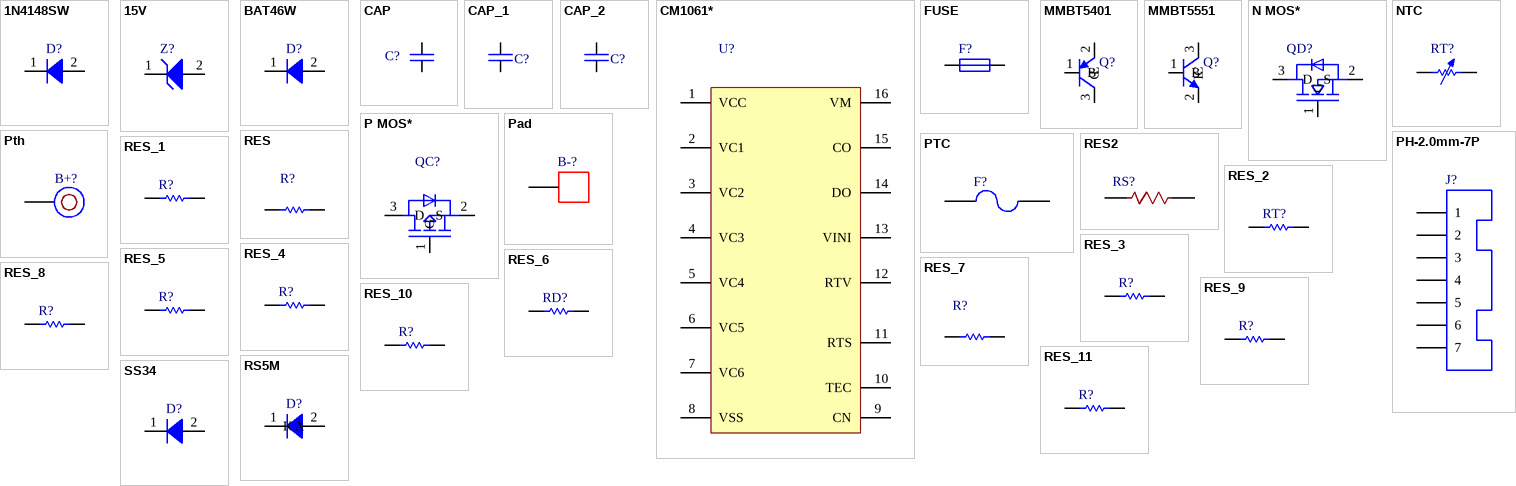
[diagram p0: symbols 1N4148SW to SS34]
# Altium schematic symbol library MISC75736.SCHLIB: 32 symbols
Pins are listed as number, name and electrical type; pins without a type are passive.


## 1N4148SW
designator D?
chip diode
footprint SOD123 (chip diode)
footprint SOD323 (chip diode)
pins: 1 A, 2    

## 15V
designator Z?
chip Zener diode
footprint SOD123 (chip diode)
footprint SOD323 (chip diode)
pins: 1 A, 2 K

## BAT46W
designator D?
chip diode
footprint SOD123 (chip diode)
footprint SOD323 (chip diode)
footprint SMAF
footprint SMC (chip diode)
pins: 1 A, 2 K

## CAP
designator C?
chip capacitor
footprint C0402A (chip capacitor)
footprint C0603A (chip capacitor)
footprint C0402L (chip resistor)
footprint C0805A (chip capacitor)
footprint C1206A (chip capacitor)
footprint C0603L (chip J-type capacitor)
footprint C0805L (chip capacitor)
footprint C0603M (chip capacitor)
pins: 1, 2

## CAP_1
designator C?
chip capacitor
footprint C0402A (chip capacitor)
footprint C0603A (chip capacitor)
footprint C0402L (chip resistor)
footprint C0805A (chip capacitor)
footprint C1206A (chip capacitor)
footprint C0603L (chip J-type capacitor)
footprint C0805L (chip capacitor)
footprint C0603M (chip capacitor)
pins: 1, 2

## CAP_2
designator C?
chip capacitor
footprint C0402A (chip capacitor)
footprint C0603A (chip capacitor)
footprint C0402L (chip resistor)
footprint C0805A (chip capacitor)
footprint C1206A (chip capacitor)
footprint C0603L (chip J-type capacitor)
footprint C0805L (chip capacitor)
footprint C0603M (chip capacitor)
pins: 1, 2

## CM1061*
designator U?
6-cell battery protection IC
footprint SOP16L
pins: 1 VCC, 2 VC1, 3 VC2, 4 VC3, 5 VC4, 6 VC5, 7 VC6, 8 VSS, 9 CN, 10 TEC, 11 RTS, 12 RTV, 13 VINI, 14 DO, 15 CO, 16 VM

## FUSE
designator F?
footprint R1206A (chip resistor)
footprint R0603A (chip resistor)
footprint R0805A (chip resistor)
footprint F2410 (chip fuse)
footprint J10*3mm (jumper 10*3mm)
pins: 1, 2

## MMBT5401
designator Q?
chip transistor
footprint SOT23-3 (chip IC/MOS*)
footprint SOT23-3L (chip MOS)
footprint SOT23-3 (chip IC/MOS*)
pins: 1 B, 2 E, 3 C

## MMBT5551
designator Q?
chip transistor
footprint SOT23-3 (chip IC/MOS*)
footprint SOT23-3L (chip MOS)
pins: 1 B, 2 E, 3 C

## N MOS*
designator QD?
chip MOSFET
footprint TO-252
footprint TO-252-DFN
footprint DFN5X6(T3)
footprint SOP-8L(T3p)
footprint DFN5X6(T3p) (chip MOS (non-standard))
footprint TO-263-TOLL
footprint DFN-3x3
footprint DFN-3x3L8(T3P) (chip MOSFET)
footprint TOLL_123 (chip MOSFET)
footprint TOLL_GSD (chip MOSFET)
pins: 1 G, 2 S, 3 D

## NTC
designator RT?
chip thermistor
footprint R0603A (chip resistor)
footprint R0402A (chip resistor)
footprint RT2.3X1-2 (wire-bond NTC)
footprint R0603L (chip resistor)
footprint R0603m (chip resistor)
footprint RT2.3X1.2-2 (wire-bond NTC)
pins: 1, 2

## P MOS*
designator QC?
chip MOSFET
footprint TOLL (chip MOSFET)
footprint TO-252
footprint TO-252-DFN
footprint DFN5X6(T3)
footprint SOP-8L(T3p)
footprint DFN5X6(T3p) (chip MOS (non-standard))
footprint TO-263-TOLL
pins: 1 G, 2 S, 3 D

## Pad
designator B-?
connection pad (non-through-hole)
footprint 3*3
footprint Pad10X8mm
footprint Pad8X6mm
pins: 1

## PH-2.0mm-7P
designator J?
connector
pins: 1, 2, 3, 4, 5, 6, 7

## PTC
designator F?
chip resettable fuse
footprint F1812A (chip resistor)
pins: 1, 2

## Pth
designator B+?
through-hole pad
footprint 4*3 (through-hole pad)
pins: 1

## RES
designator R?
chip resistor
footprint R0603A (chip resistor)
footprint R0201A
footprint R0402A (chip resistor)
footprint R0603m (chip resistor)
footprint R0805A (chip resistor)
footprint R0402L (chip resistor)
footprint RES0603 (CAP0402)
footprint R0603L (chip resistor)
footprint R0805L (chip resistor)
footprint R0805M (chip resistor)
footprint R1206A (chip resistor)
pins: 1, 2

## RES2
designator RS?
chip metal alloy resistor
footprint R2512L (chip resistor)
pins: 1, 2

## RES_1
designator R?
chip resistor
footprint R0603A (chip resistor)
footprint R0201A
footprint R0402A (chip resistor)
footprint R0603m (chip resistor)
footprint R0805A (chip resistor)
footprint R0402L (chip resistor)
footprint RES0603 (CAP0402)
footprint R0603L (chip resistor)
footprint R0805L (chip resistor)
footprint R0805M (chip resistor)
footprint R1206A (chip resistor)
pins: 1, 2

## RES_2
designator RT?
chip resistor
footprint R0603A (chip resistor)
footprint R0201A
footprint R0402A (chip resistor)
footprint R0603m (chip resistor)
footprint R0805A (chip resistor)
footprint R0402L (chip resistor)
footprint RES0603 (CAP0402)
footprint R0603L (chip resistor)
footprint R0805L (chip resistor)
footprint R0805M (chip resistor)
footprint R1206A (chip resistor)
pins: 1, 2

## RES_3
designator R?
chip resistor
footprint R0603A (chip resistor)
footprint R0201A
footprint R0402A (chip resistor)
footprint R0603m (chip resistor)
footprint R0805A (chip resistor)
footprint R0402L (chip resistor)
footprint RES0603 (CAP0402)
footprint R0603L (chip resistor)
footprint R0805L (chip resistor)
footprint R0805M (chip resistor)
footprint R1206A (chip resistor)
pins: 1, 2

## RES_4
designator R?
chip resistor
footprint R0603A (chip resistor)
footprint R0201A
footprint R0402A (chip resistor)
footprint R0603m (chip resistor)
footprint R0805A (chip resistor)
footprint R0402L (chip resistor)
footprint RES0603 (CAP0402)
footprint R0603L (chip resistor)
footprint R0805L (chip resistor)
footprint R0805M (chip resistor)
footprint R1206A (chip resistor)
pins: 1, 2

## RES_5
designator R?
chip resistor
footprint R0603A (chip resistor)
footprint R0201A
footprint R0402A (chip resistor)
footprint R0603m (chip resistor)
footprint R0805A (chip resistor)
footprint R0402L (chip resistor)
footprint RES0603 (CAP0402)
footprint R0603L (chip resistor)
footprint R0805L (chip resistor)
footprint R0805M (chip resistor)
footprint R1206A (chip resistor)
pins: 1, 2

## RES_6
designator RD?
chip resistor
footprint R0603A (chip resistor)
footprint R0201A
footprint R0402A (chip resistor)
footprint R0603m (chip resistor)
footprint R0805A (chip resistor)
footprint R0402L (chip resistor)
footprint RES0603 (CAP0402)
footprint R0603L (chip resistor)
footprint R0805L (chip resistor)
footprint R0805M (chip resistor)
footprint R1206A (chip resistor)
pins: 1, 2

## RES_7
designator R?
chip resistor
footprint R0603A (chip resistor)
footprint R0201A
footprint R0402A (chip resistor)
footprint R0603m (chip resistor)
footprint R0805A (chip resistor)
footprint R0402L (chip resistor)
footprint RES0603 (CAP0402)
footprint R0603L (chip resistor)
footprint R0805L (chip resistor)
footprint R0805M (chip resistor)
footprint R1206A (chip resistor)
pins: 1, 2

## RES_8
designator R?
chip resistor
footprint R0603A (chip resistor)
footprint R0201A
footprint R0402A (chip resistor)
footprint R0603m (chip resistor)
footprint R0805A (chip resistor)
footprint R0402L (chip resistor)
footprint RES0603 (CAP0402)
footprint R0603L (chip resistor)
footprint R0805L (chip resistor)
footprint R0805M (chip resistor)
footprint R1206A (chip resistor)
pins: 1, 2

## RES_9
designator R?
chip resistor
footprint R0603A (chip resistor)
footprint R0201A
footprint R0402A (chip resistor)
footprint R0603m (chip resistor)
footprint R0805A (chip resistor)
footprint R0402L (chip resistor)
footprint RES0603 (CAP0402)
footprint R0603L (chip resistor)
footprint R0805L (chip resistor)
footprint R0805M (chip resistor)
footprint R1206A (chip resistor)
pins: 1, 2

## RES_10
designator R?
chip resistor
footprint R0603A (chip resistor)
footprint R0201A
footprint R0402A (chip resistor)
footprint R0603m (chip resistor)
footprint R0805A (chip resistor)
footprint R0402L (chip resistor)
footprint RES0603 (CAP0402)
footprint R0603L (chip resistor)
footprint R0805L (chip resistor)
footprint R0805M (chip resistor)
footprint R1206A (chip resistor)
pins: 1, 2

## RES_11
designator R?
chip resistor
footprint R0603A (chip resistor)
footprint R0201A
footprint R0402A (chip resistor)
footprint R0603m (chip resistor)
footprint R0805A (chip resistor)
footprint R0402L (chip resistor)
footprint RES0603 (CAP0402)
footprint R0603L (chip resistor)
footprint R0805L (chip resistor)
footprint R0805M (chip resistor)
footprint R1206A (chip resistor)
pins: 1, 2

## RS5M
designator D?
chip diode
footprint SMAF
footprint SMB(DO-214AA) (chip diode)
footprint SMC A(DO-214AB) (chip diode)
pins: 1 A, 2 K

## SS34
designator D?
chip Schottky diode
footprint SMA(DO-214AC) (chip diode)
footprint SMB(DO-214AA) (chip diode)
footprint SMB_M(DO-214AA) (chip diode)
pins: 1 A, 2 K